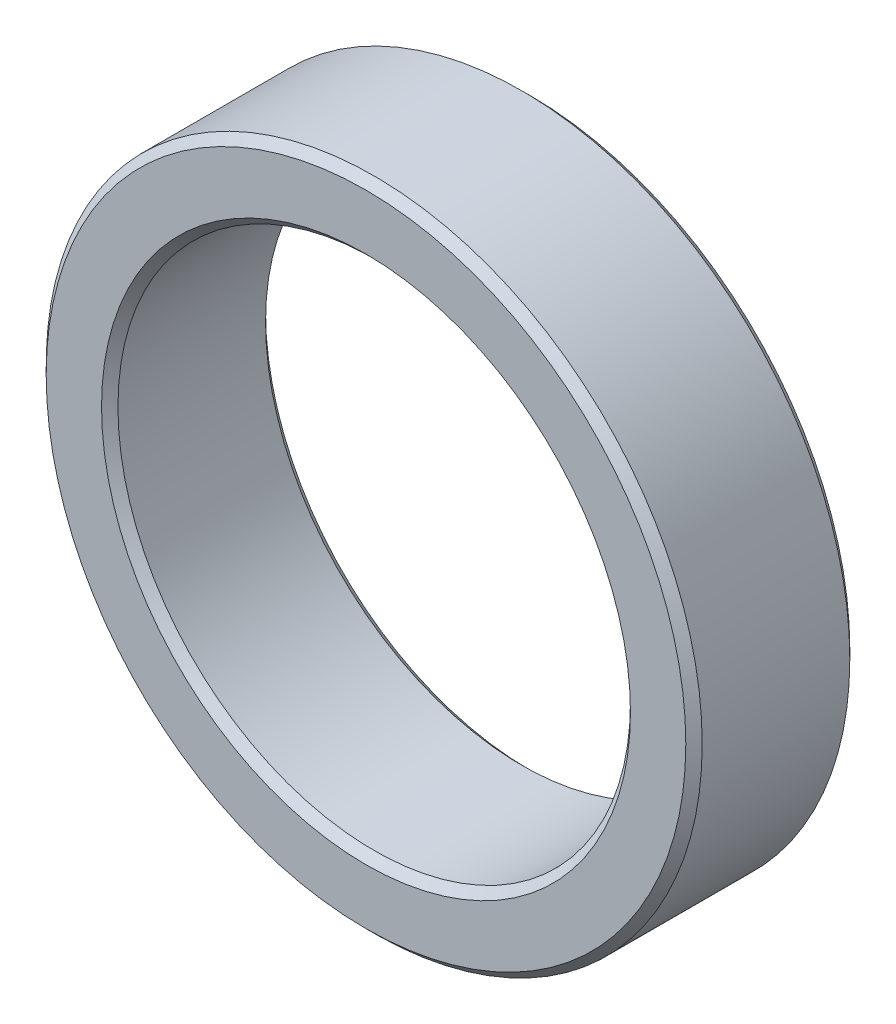
from build123d import *

# Parameters (mm, degrees)
SKETCH1_R           = 8
SKETCH1_R_2         = 6.25
BOSS_EXTRUDE1_DEPTH = 2
CHAMFER1_SIZE       = 0.2


with BuildPart() as part:
    # Sketch1 → Boss-Extrude1 (new, symmetric)
    with BuildSketch(Plane.XY):
        Circle(SKETCH1_R)
        Circle(SKETCH1_R_2, mode=Mode.SUBTRACT)
    extrude(amount=BOSS_EXTRUDE1_DEPTH, both=True)

    # Chamfer1
    chamfer1_edges = [part.edges().sort_by_distance(p)[0] for p in [
        (-8, 0, -2),
        (-8, 0, 2),
        (-6.25, 0, -2),
        (-6.25, 0, 2),
    ]]
    chamfer(chamfer1_edges, length=CHAMFER1_SIZE)


solid = part.part
